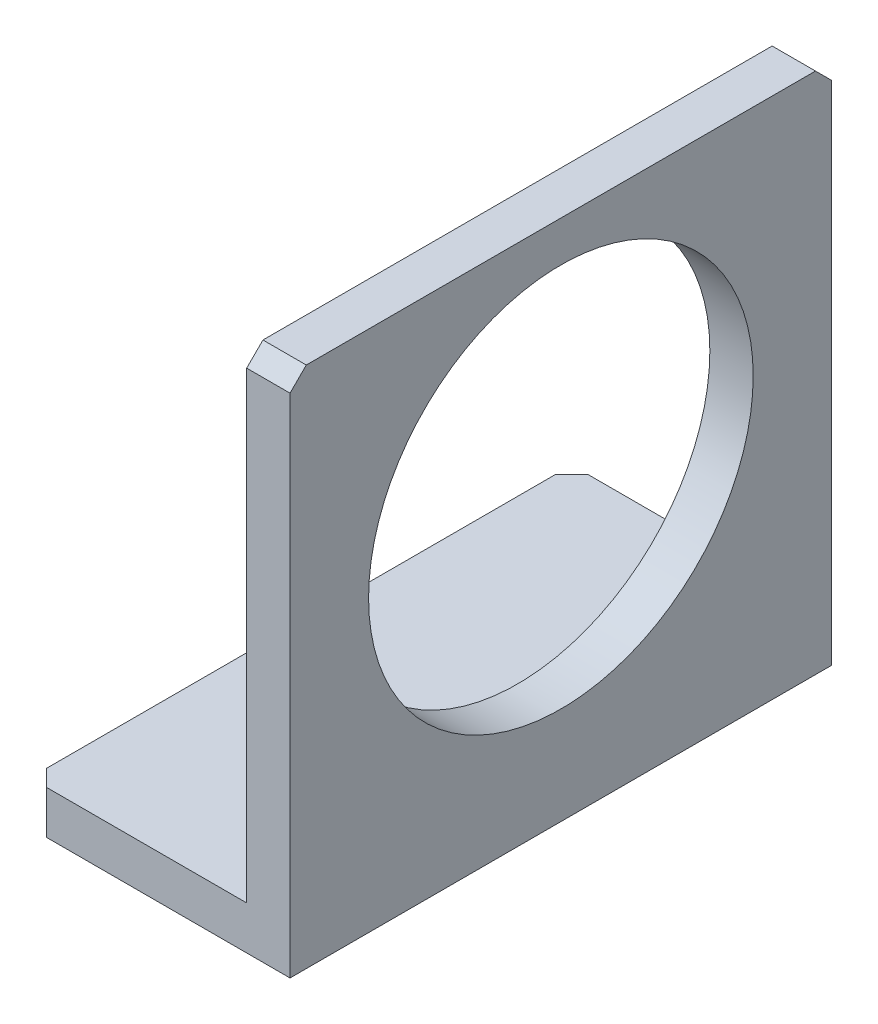
SolidWorks part; units mm, degrees
ref_plane "前视基准面" through (0, 0, 0) normal (0, 0, 1) x (1, 0, 0)
ref_plane "上视基准面" through (0, 0, 0) normal (0, 1, 0) x (1, 0, 0)
ref_plane "右视基准面" through (0, 0, 0) normal (1, 0, 0) x (0, 0, -1)
sketch "草图2" plane through (409.6376, 0.5, -34.3795) normal (0, 0, 1) x (1, 0, 0)
  line L0 (-409.6376, 96) -> (-409.6376, -0.5)
  line L1 (-409.6376, -0.5) -> (-457.6376, -0.5)
  line L2 (-457.6376, -0.5) -> (-457.6376, 7.5)
  line L3 (-457.6376, 7.5) -> (-417.6376, 7.5)
  line L4 (-417.6376, 7.5) -> (-417.6376, 96)
  line L5 (-417.6376, 96) -> (-409.6376, 96)
  dimension "D2" = 8
  dimension "D3" = 8
  dimension "D4" = 88.5
  dimension "D5" = 40
extrude "凸台-拉伸1" add sketch "草图2" along normal mid plane 100
chamfer "倒角1" distance 3 angle 45 4 edges at (-48, 4, -84.3795) (-48, 4, 15.6205) (-4, 96.5, 15.6205) (-4, 96.5, -84.3795)
sketch "草图4" plane through (-8, 0, 0) normal (-1, 0, 0) x (0, 0, 1)
  line L0 (-34.3795, 53.5) -> (-34.3795, 96.5) construction
  line L1 (12.6205, 96.5) -> (-81.3795, 96.5) construction
  circle A0 centre (-34.3795, 53.5) radius 35.5
  dimension "D2" = 71
  dimension "D1" = 43
extrude "切除-拉伸1" cut sketch "草图4" against normal up to next
